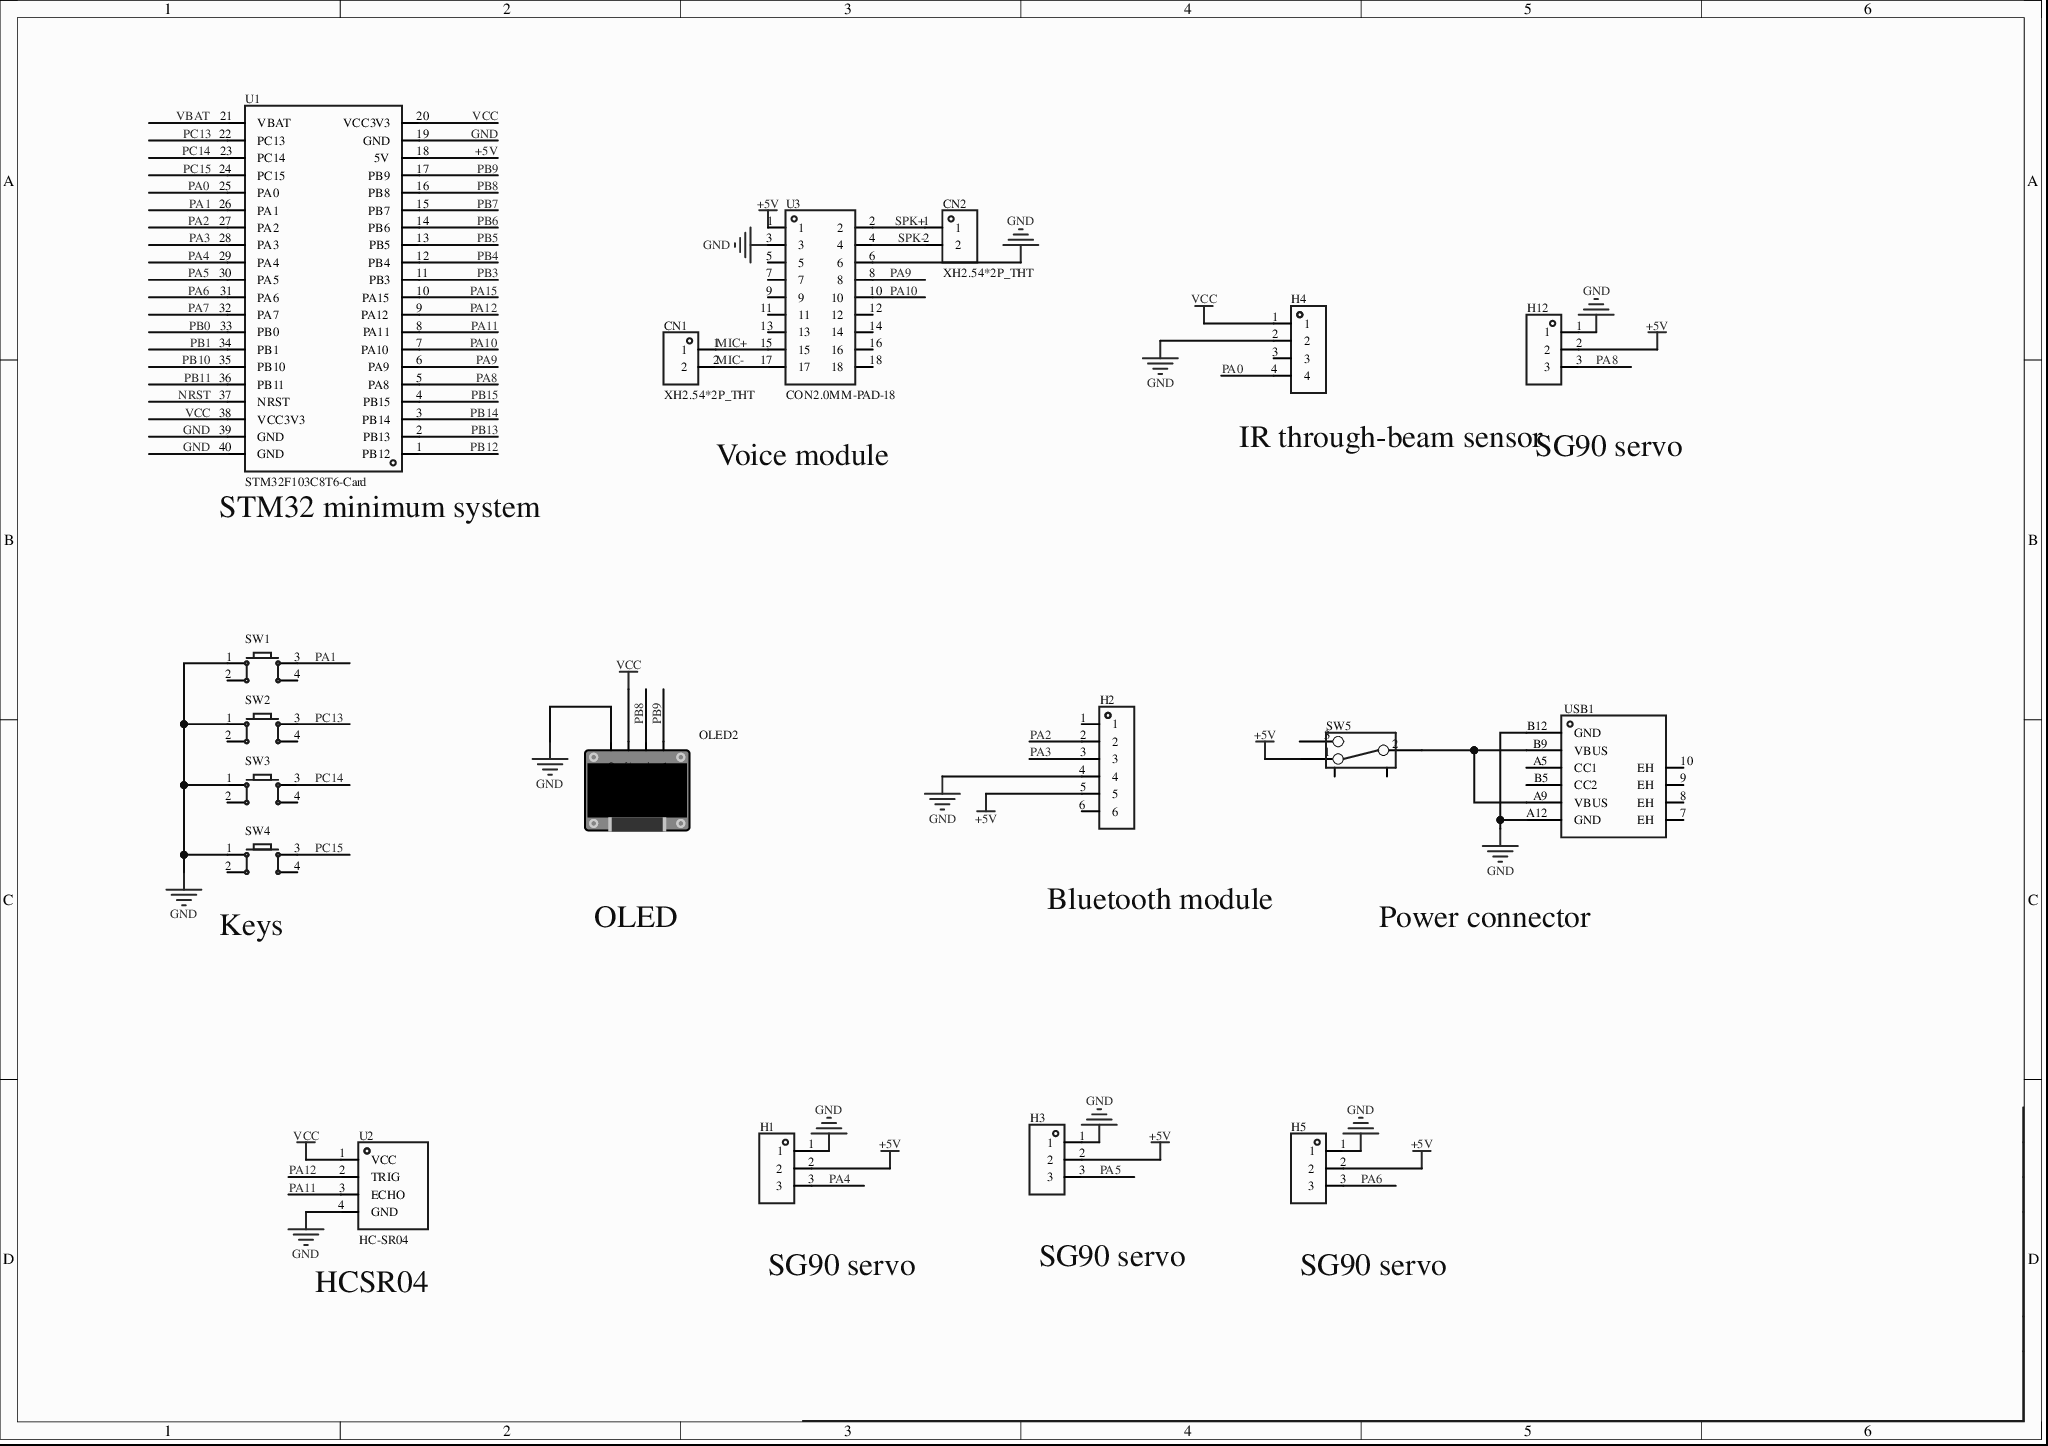
[diagram p0: MISC51947-3.schdoc]
# Altium project MISC51947-2.PrjPcb
1 sheet, 18 parts. Net scope: global (net labels, ports and power ports of the same name join across sheets).
Board file: MISC51947.pcbdoc

## Sheet MISC51947-3.schdoc
size 297 x 209 mm; Version: V1.0; @Project Name: MISC51947; @Page Count: 1; @Update Date: 2026-05-06; @Create Date: 2026-05-06; @Schematic Name: MISC51947; @Page No: 1; @Create Time: 23:22:16; @Update Time: 17:32:40; @Board Name: MISC51947

### Parts
CN1  XH2.54*2P_THT  [CONN-TH_2P-P2.50-XH2.54-2P]
CN2  XH2.54*2P_THT  [CONN-TH_2P-P2.50-XH2.54-2P]
H1  (no value)  [HDR-TH_3P-P2.54-V-F]
H2  (no value)  [HDR-TH_6P-P2.54-V-F]
H3  (no value)  [HDR-TH_3P-P2.54-V-F]
H4  (no value)  [HDR-TH_4P-P2.54-V-F]
H5  (no value)  [HDR-TH_3P-P2.54-V-F]
H12  (no value)  [HDR-TH_3P-P2.54-V-F]
OLED2  (no value)  [0.96OLED_4P]
SW1  (no value)  [SW-TH_4P-L6.0-W6.0-P4.50-LS6.5]
SW2  (no value)  [SW-TH_4P-L6.0-W6.0-P4.50-LS6.5]
SW3  (no value)  [SW-TH_4P-L6.0-W6.0-P4.50-LS6.5]
SW4  (no value)  [SW-TH_4P-L6.0-W6.0-P4.50-LS6.5]
SW5  (no value)  [拨动开关]
U1  STM32F103C8T6-Card  [CONN-TH_L53.3-W22.9_STM32F103C8T6-CARD]
U2  HC-SR04  [TH_HC-SR04V]
U3  CON2.0MM-PAD-18  [CONN-TH_18P-P2.00_C9900078766]
USB1  (no value)  [USB_ TYPE-C-6P]

### Nets
+5V: H1.2 H2.5 H3.2 H5.2 H12.2 SW5.1 U1.18(5V) U3.1
GND: H1.1 H2.4 H3.1 H4.2 H5.1 H12.1 OLED2.1(GND) SW1.1 SW2.1 SW3.1 SW4.1 U1.19(GND) U1.39(GND) U1.40(GND) U2.4(GND) U3.3 U3.6 USB1.A12(GND) USB1.B12(GND)
VCC: H4.1 OLED2.2(VCC) U1.20(VCC3V3) U1.38(VCC3V3) U2.1(VCC)
MIC+: CN1.1 U3.15
MIC-: CN1.2 U3.17
NRST: U1.37(NRST)
PA0: H4.4 U1.25(PA0)
PA1: SW1.3 U1.26(PA1)
PA2: H2.2 U1.27(PA2)
PA3: H2.3 U1.28(PA3)
PA4: H1.3 U1.29(PA4)
PA5: H3.3 U1.30(PA5)
PA6: H5.3 U1.31(PA6)
PA7: U1.32(PA7)
PA8: H12.3 U1.5(PA8)
PA9: U1.6(PA9) U3.8
PA10: U1.7(PA10) U3.10
PA11: U1.8(PA11) U2.3(ECHO)
PA12: U1.9(PA12) U2.2(TRIG)
PA15: U1.10(PA15)
PB0: U1.33(PB0)
PB1: U1.34(PB1)
PB3: U1.11(PB3)
PB4: U1.12(PB4)
PB5: U1.13(PB5)
PB6: U1.14(PB6)
PB7: U1.15(PB7)
PB8: OLED2.3(SCL) U1.16(PB8)
PB9: OLED2.4(SDA) U1.17(PB9)
PB10: U1.35(PB10)
PB11: U1.36(PB11)
PB12: U1.1(PB12)
PB13: U1.2(PB13)
PB14: U1.3(PB14)
PB15: U1.4(PB15)
PC13: SW2.3 U1.22(PC13)
PC14: SW3.3 U1.23(PC14)
PC15: SW4.3 U1.24(PC15)
SPK+: CN2.1 U3.2
SPK-: CN2.2 U3.4
VBAT: U1.21(VBAT)
NetSW5_2: SW5.2 USB1.A9(VBUS) USB1.B9(VBUS)

Not connected (* = marked no-connect by the designer): H2 1 6; H4 3; SW1 2 4; SW2 2 4; SW3 2 4; SW4 2 4; SW5 3 4 5; U3 5 7 9 11 12 13 14 16 18; USB1 7(EH) 8(EH) 9(EH) 10(EH) A5(CC1) B5(CC2)

### Notes on the sheet
- 语音识别：LD3320➕语音播报JQ8900-16P
  满溢检测：红外对射管
  执行机构：SG90 舵机
  备用控制：4 路独立按键
  显示模块：0.96 寸OLED (IIC)
  无线通信：JDY31 蓝牙模块
  供电模块：USB 5V/2A
  火情监测：HCSR04 超声波
- (near U1) STM32 minimum system
- Voice module
- IR through-beam sensor
- (near H12) SG90 servo
- (near SW4) Keys
- OLED
- Bluetooth module
- Power connector
- (near U2) HCSR04
- (near H1) SG90 servo
- (near H3) SG90 servo
- (near H5) SG90 servo

### Library data of the parts
CN1 CN2 = XH2.54*2P_直插: 3D Model: 325c595e30db4df8abe76612dd40b0fa0819f05c4eef4c71ace90d822a990e87; 3D Model Transform: 295.275,228.346,0,180,0,0,-0.002,-20.079,-137.795; AddInBom: yes; Symbol: XH2.54*2P_THT; Device: XH2.54*2P_THT; LCSC Part Name: XH2.54*2P_直插; Supplier Part: C9900008615; Manufacturer Part: XH2.54*2P_直插; Supplier Footprint: XH2.54_2P; JLCPCB Part Class: Extended Part; Supplier: LCSC; ConvertToPcb: yes; FootprintName: CONN-TH_2P-P2.50-XH2.54-2P; ModelName: CONN-TH_2P-P2.50-XH2.54-2P
H1 H3 H5 H12 = HDR-F_2.54_1x3P: Symbol: PM254V-11-03-H85; 3D Model: f3b3cc5aae9641bf9e56fc160cef875b; 3D Model Transform: 299.9994,100,0,0,0,0,0,0,-118.11; ConvertToPcb: yes; ModelName: HDR2.54-F-LI-1X3P; Device: HDR-F_2.54_1x3P; Supplier Part: C541850; Supplier Footprint: 插件; FootprintName: HDR-TH_3P-P2.54-V-F; AddInBom: yes
H2 = HDR-F_2.54_1x6P: Symbol: Header-Female-2.54_1x6; ConvertToPcb: yes; ModelId: 0f5bcf94dcda47d085f24cdca1696fe9; ModelTransform: 619.684,94.488,0,0,0,0,0,0,-125.984; Device: HDR-F_2.54_1x6P; AddInBom: yes; SupplierPart: C40877; Supplier Footprint: 插件; FootprintName: HDR-TH_6P-P2.54-V-F; ModelName: HDR-TH_6P-P2.54-V-F
H4 = HDR-F_2.54_1x4P: Symbol: 2.54-1*4P female; ConvertToPcb: yes; ModelId: d187812051054f85879fcaa51a310d8e0819f05c4eef4c71ace90d822a990e87; ModelTransform: 419.6842,98.464,0,0,0,0,0,0,-118.11; Device: HDR-F_2.54_1x4P; FootprintName: HDR-TH_4P-P2.54-V-F; AddInBom: yes; SupplierPart: C2718488; Supplier Footprint: 插件; ModelName: HDR-TH_4P-P2.54-V-F
OLED2 = 0.96OLED模块_4P: Symbol: 0.96OLED module_4P; ConvertToPcb: yes; ModelId: 79c000fdb68d45a296c2e9bedf4f9055; ModelTransform: 1393.69792,1318.895,0,0,0,0,0,-560.079,-137.795; Device: 0.96OLED module_4P; AddInBom: yes; FootprintName: 0.96OLED_4P; Supplier Footprint: 插件; ModelName: 0.96OLED_4P
SW1-SW4 = Key_TH_6x6x6: Contact current:50mA; rated voltage (DC):12V; insulation resistance:100MΩ; circuit:SPST; mounting:through-hole; button shape:round; button/cap color:black; actuating force:260gf@±30gf; operating temperature:-25℃~+70℃; pin style:PC pin; switch length:6mm; switch width:6mm; switch height:6mm; with bracket:no;; Symbol: Tactile key; AddInBom: yes; ModelId: 20eee248bc684ccd8cbdbb1d0d91ec6f0819f05c4eef4c71ace90d822a990e87; ModelName: SW-TH_4P-L6.0-W6.0-H5.0-LS6.5-P4.50; ModelTransform: 236.22,323.03,0,90,0,0,0,0,-137.795; Device: Key_TH_6x6x6; FootprintName: SW-TH_4P-L6.0-W6.0-P4.50-LS6.5; ConvertToPcb: yes; Supplier Footprint: 插件
SW5 = 拨动开关_正: Device: Toggle switch_pos; Symbol: Toggle switch; ConvertToPcb: yes; ModelId: 4321fe59a4074cbfb4989553f297c68f0819f05c4eef4c71ace90d822a990e87; ModelName: SW-TH_SS-12D02-VG4; ModelTransform: 370.09,208.7,472.35,0,0,0,0,0,-110; FootprintName: Toggle switch; AddInBom: yes; Supplier Footprint: 插件
U1 = STM32F103C8T6-Card: AddInBom: yes; Device: STM32F103C8T6-Card; Symbol: STM32F103C8T6-CARD; FootprintName: CONN-TH_L53.3-W22.9_STM32F103C8T6-CARD; LCSC Part Name: STM32F103C8T6-Card; SupplierPart: C9900077949; ManufacturerPart: STM32F103C8T6-Card; Supplier Footprint: 插件; Supplier: LCSC; ConvertToPcb: yes
U2 = HC-SR04: Manufacturer: Universal Microelectronics; AddInBom: yes; Symbol: HC-SR04; Device: HC-SR04; LCSC Part Name: HC-SR04; SupplierPart: C19857336; ManufacturerPart: HC-SR04; Supplier Footprint: -; JLCPCB Part Class: Extended library; Datasheet: https://atta.szlcsc.com/upload/public/pdf/source/20240122/47B8E374E428935B7962A2189EF91AAC.pdf; Supplier: LCSC; ConvertToPcb: yes; FootprintName: TH_HC-SR04V
U3 = CON2.0MM-PAD-18: 3D Model: 07100c6dd3a4442ea12d6f5a4e41c4c80819f05c4eef4c71ace90d822a990e87; 3D Model Transform: 787.7937,374.015,0,0,0,0,0,-14.961,-118.11; AddInBom: yes; Symbol: CON2.0MM-PAD-18; Device: CON2.0MM-PAD-18; LCSC Part Name: CON2.0MM-PAD-18; Supplier Part: C9900078766; Manufacturer Part: CON2.0MM-PAD-18; Supplier Footprint: TH-2*9P-2.0; JLCPCB Part Class: Extended Part; Supplier: LCSC; ConvertToPcb: yes; FootprintName: CONN-TH_18P-P2.00_C9900078766; ModelName: CONN-TH_18P-P2.00_C9900078766
USB1 = USB_ Type-C-6P: AddInBom: yes; ModelId: d4f492a4e6024845a13b3f6a4ef2d2cb0819f05c4eef4c71ace90d822a990e87; ModelName: USB-SMD_U262-061N-4BVC11; ModelTransform: 352.362,281.496,0,0,0,0,0,-47.244,-39.37; Symbol: USB_ TYPE-C-6P; Device: USB_ Type-C-6P; Supplier Footprint: SMD; ConvertToPcb: yes; FootprintName: USB_ TYPE-C-6P